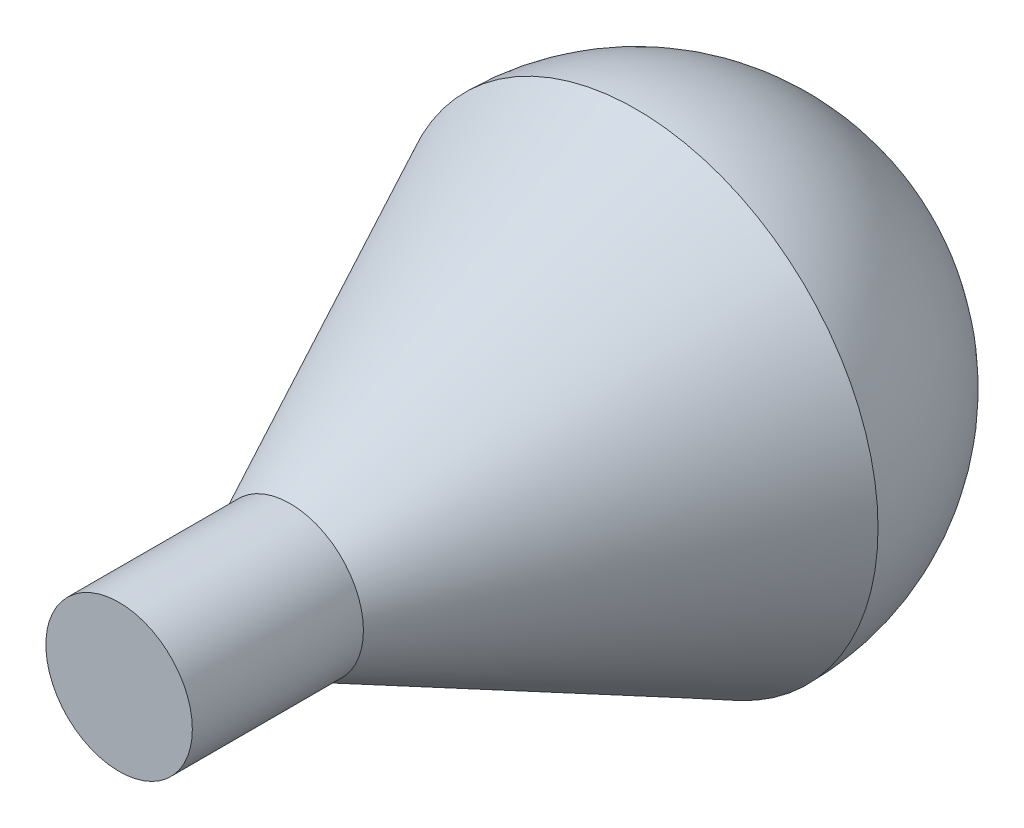
from build123d import *


with BuildPart() as part:
    # Sketch1 → Revolve1 (revolve)
    with BuildSketch(Plane(origin=(0, 0, 0), x_dir=(1, 0, 0), z_dir=(0, 1, 0))):
        with BuildLine():
            Line((0, 0), (7.239896535, 0))
            Line((7.239896535, 0), (7.239896535, 16.912213927))
            Line((7.239896535, 16.912213927), (23.910442474, 51.11198251))
            ThreePointArc((23.910442474, 51.11198251), (16.907236015, 68.019218524), (0, 75.022424984))
            Line((0, 75.022424984), (0, 51.11198251))
            Line((0, 51.11198251), (0, 0))
        make_face()
    revolve(axis=Axis((0, 0, -51.11198251), (0, 0, -1)))


solid = part.part
